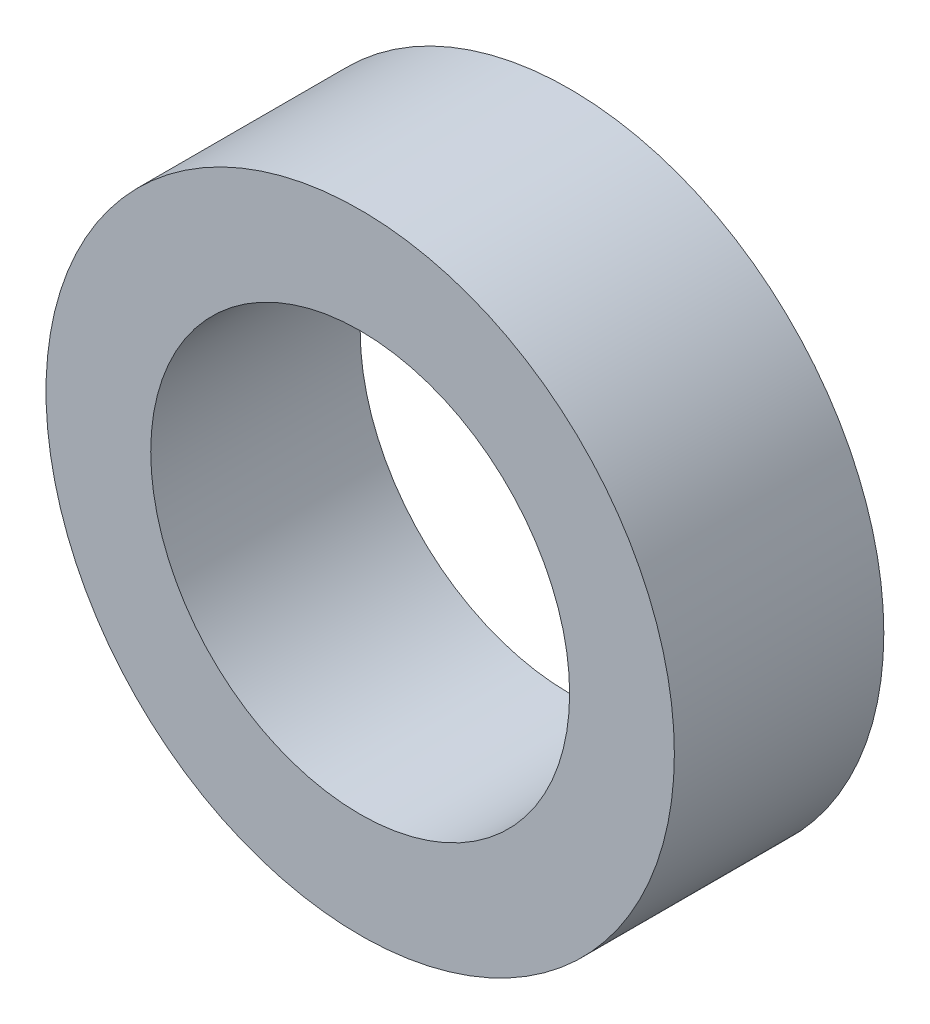
SolidWorks part; units mm, degrees
ref_plane "Front Plane" through (0, 0, 0) normal (0, 0, 1) x (1, 0, 0)
ref_plane "Top Plane" through (0, 0, 0) normal (0, 1, 0) x (1, 0, 0)
ref_plane "Right Plane" through (0, 0, 0) normal (1, 0, 0) x (0, 0, -1)
sketch "Sketch1" plane through (0, 0, 0) normal (0, 0, 1) x (1, 0, 0)
  circle A0 centre (0, 0) radius 2
  circle A1 centre (0, 0) radius 3
  dimension "D1" = 4
  dimension "D2" = 6
extrude "Boss-Extrude1" add sketch "Sketch1" along normal blind 2
